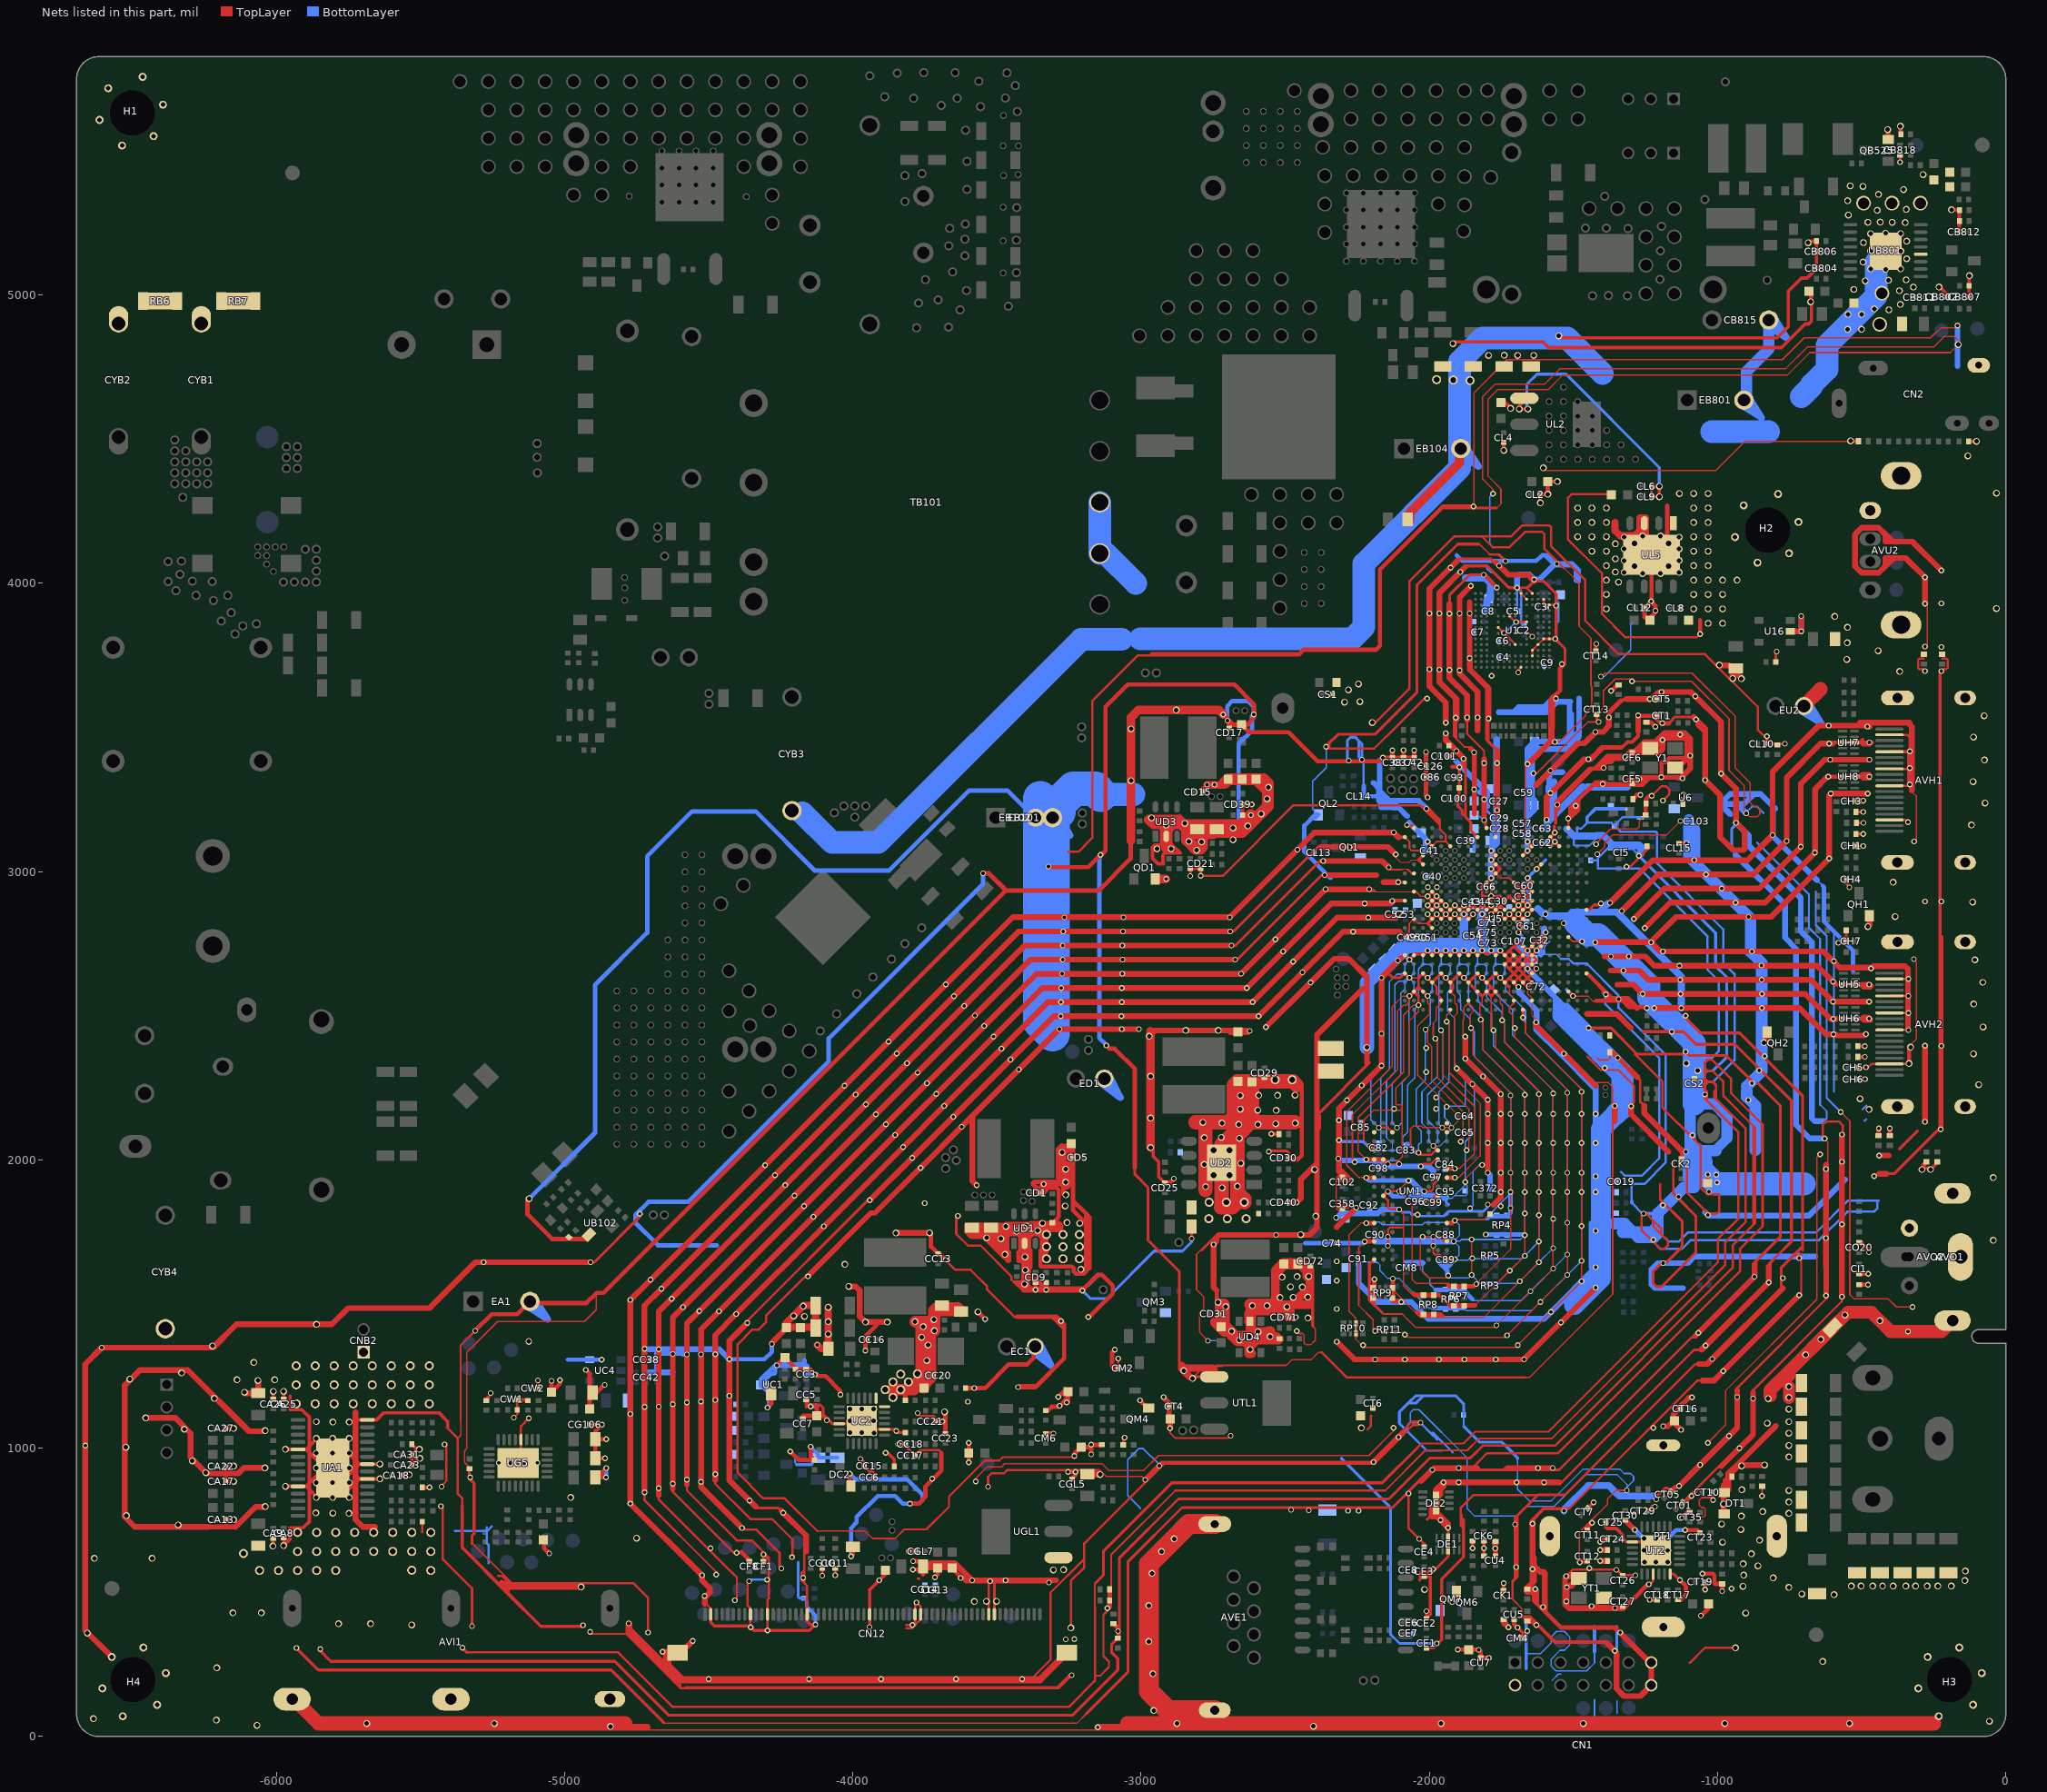
[diagram p0: the nets of this part, all layers, seen from the top]
# Altium PCB MISC84395.PcbDoc (part 16 of 26)
Units mil, origin at the board's own origin, x right, y up, seen from the top; angles counter-clockwise.
Board outline 6692.91 x 5826.77 mil, 2 copper layers (TopLayer, BottomLayer), stack 61.855 mil thick; 951 components, 565 nets, 4374 pads, 1804 vias.
Unrouted connection lines stored in the file: 1.

## Via types
v1: diameter 19.68, hole 11.81, TopLayer to BottomLayer, tented both sides, 1262 vias
v2: diameter 23.62, hole 15.75, TopLayer to BottomLayer, tented both sides, 524 vias
v3: diameter 31.5, hole 19.68, TopLayer to BottomLayer, tented both sides, 11 vias
v4: diameter 24, hole 16, TopLayer to BottomLayer, tented both sides, 6 vias
v5: diameter 19, hole 11.81, TopLayer to BottomLayer, tented both sides, 1 vias

## Nets (pads, with @x,y where several pads share a name; then routed paths per layer and width w, separated by ;. In a path a pad name is that pad's centre, name@x,y a point inside that pad or via, vN(x,y) a via of type N, cw(c..) or ccw(c..) an arc to the next point about the centre after c; other vN are vias at no path point) (continued)
GND: (continued)
  TopLayer w12: v2(-6011.23,661) -6011.23,687.54 CA9.1@-6010.23,688.54 ; CA26.1@-6010.52,1169.98 -6010.52,1196.71 v2(-6010.23,1197) v2@-6009.23,1196 ; v2@-5975.64,663.41 v2(-5974.23,662) ; v2@-5975.23,1196 v2(-5974.23,1197) -5974.17,1196.94 CA25.2@-5974.17,1169.96 ; CA8.1@-5974.23,688.8 v2@-5974.23,662 ; -5952.23,1181.3 -5952.23,1134.04 -5952.19,1134 -5911.57,1134 -5885.23,1107.67 -5885.23,1007.2 ; UA1.24@-5924.23,867.96 -5896.52,867.96 ; UA1.19@-5924.23,995.92 -5896.52,995.92 ; v2@-5858.13,829.58 -5885.23,856.68 ; UA1.EPAD@-5858.13,906.35 -5885.23,879.25 ; UA1.EPAD@-5858.13,957.53 -5885.23,984.63 ; v2@-5858.13,1034.3 -5885.23,1007.2 ; v2(-5804.15,931.94) -5750.17,931.94 -5748.62,930.39 -5737.38,919.15 ; UA1.EPAD@-5750.17,855.17 -5724.67,880.68 -5711.79,893.55 ; UA1.EPAD@-5750.17,906.35 -5737.38,919.15 ; UA1.EPAD@-5750.17,983.12 -5724.67,957.61 -5711.79,944.74 ; -5711.79,1098.28 UA1.14@-5684.07,1098.28 -5651.67,1098.28 -5626.94,1123 -5436.47,1123 -5405.1,1091.63 -5405.1,1074.37 -5406.41,1073.06 ; v2@-5642.04,946.81 v2(-5640.23,945) -5640.5,944.74 UA1.8@-5684.07,944.74 -5711.79,944.74 ; v2@-5640.29,894.06 v2(-5640.23,894) -5640.68,893.55 UA1.6@-5684.07,893.55 -5711.79,893.55 ; CA18.2@-5566.5,906 -5541.23,906 v2(-5539.23,908) -5553.23,908 ; RA21.1@-5529.86,1013.94 -5510.57,994.65 -5513.15,994.65 CA31.2@-5529.86,977.94 CA23.2@-5529.86,941.94 -5511.86,959.94 v2@-5506.56,959.94 ; RA19.1@-5493.86,863.94 -5468.29,863.94 v1(-5468.23,864) ; v1@-5429.23,864 v1(-5426.23,867) ; -5355.07,798.5 -5355.07,655.07 -5195,495 ; -5197.39,537.61 -5196.5,536.72 -5196.5,496.5 -5195,495 ; v1(-4936,386) -4940,382 -5082,382 -5195,495 ; -3941.85,508.15 v1(-3908,542) -3887.19,562.81 CG12.1@-3887.19,577 ; v1(-3886,984) -3883,987 -3882.24,987 -3856.27,961.02 RC26.1@-3856.27,937 ; RM9.2@-3062,1011.73 -3060.5,1013.23 -3060.5,1033.5 v1(-3057.5,1036.5) ; v2(-2967,2043) -2958,2034 -2958,2012.44 -2939,1993.44 -2939,1941.89 CD25.1@-2917,1919.89 ; -2854.76,3123 -2854.76,3140.48 -2866.97,3152.69 -2884.23,3152.69 -2896.44,3140.48 -2896.44,3096.4 -2864.47,3064.43 -2917.66,3064.43 -2924.1,3057.98 -2924.1,3031.15 -2921.62,3028.67 -2921.62,3027 -2941.72,3027 -2960.25,3045.53 -2960.25,3084.07 -2953,3091.32 -2936,3091.32 -2929.56,3097.77 -2929.56,3146.25 -2936,3152.69 -2961.29,3152.69 -2984.16,3175.56 -2984.16,3185 -2977.16,3192 -2868.65,3192 -2866.55,3194.1 -2848,3175.56 pad.VIA5@-2848,3166.69 ; RD16.1@-2829.26,3010.98 CD21.2@-2793.26,3010.97 ; RD27.2@-2647.56,3195.87 CD39.2@-2647.56,3232.87 ; UM1.J2@-2159.73,1875.45 v1(-2143.99,1891.2) ; v1@-2124.91,2899.08 U5.N21@-2084.93,2899.08 ; -2101.84,3119.55 U5.Y21@-2084.93,3119.55 ; -2097.64,2787.76 -2084.93,2775.05 U5.J21@-2084.93,2773.09 ; -2061.17,3158.78 -2060.39,3158 ; C101.2@-1931.91,3399.74 -1924.65,3399.74 v1(-1906.07,3418.31) ; v1(-1921,466) -1906.5,480.5 QM6.E@-1906.5,504 ; -1918.27,3363.45 -1917.48,3363.45 ; v1(-1850,653) R37.1@-1850,678.27 ; DK3.A@-1811,626.73 v1(-1811,653) CK6.1@-1811,678.27 ; CU4.1@-1771,623.73 CU4.1@-1770.01,624.71 ; CL3.2@-1746,4633.81 CL3.2@-1743.32,4633.81 ; CK1.2@-1743,506.74 v1@-1743,530.38 ; v1@-1743,532 v1@-1743,530.38 ; v2@-1742,4461 CL4.2@-1742,4488.26 ; v1(-1741.94,531.44) v1@-1743,530.38 ; CL3.2@-1739.32,4633.81 CL3.2@-1743.32,4633.81 ; v2@-1718.32,4608.81 CL3.2@-1743.32,4633.81 ; v1(-1694.06,378.06) -1677,361 CM4.1@-1677,350 ; CM4.1@-1677,341 CM4.1@-1677,350 ; -1675.5,414.99 -1674.71,414.2 -1670.94,414.2 -1650.8,414.2 v1@-1625.95,389.35 ; UL2.1@-1666.54,4641.55 -1666.54,4637.46 -1688,4616 v2(-1688,4604) v2(-1658,4604) ; v1(-1660,366) -1661,366 CM4.1@-1677,350 ; v1@-1646.5,746.54 -1603.04,790 -1540,790 v1(-1533,783) ; v1@-1634.73,510.73 -1638.17,507.29 -1638.17,496.34 -1638.17,470.88 -1549.69,382.39 -1543.69,376.39 -1535.69,376.39 -1516,376.39 ; v1@-1628.88,392.29 v1@-1625.95,389.35 ; v2(-1615,4279) -1616.26,4280.26 CL2.2@-1616.26,4308 -1590,4308 -1589.19,4308.81 v2(-1589,4309) ; CL1.1@-1589.19,4352 -1556.63,4352 v2(-1555.63,4353) ; -1533.5,547.52 -1533.5,457.65 -1522.35,446.5 -1358.23,446.5 -1334.06,446.5 CT27.1@-1329.29,451.27 -1363,451.27 -1424.96,451.27 -1436.05,451.27 v1(-1437.03,452.26) ; U5.C3@-1518,2584.12 -1517.68,2584.12 v1(-1502.25,2568.68) ; CT7.1@-1450.21,791.79 v1(-1430,812) ; CT14.2@-1422,3764.74 -1422,3789 v1(-1421,3790) ; v1@-1407.46,608.54 v1(-1407,609) ; v1(-1407.29,675) -1398.31,683.98 CT24.2@-1381.81,683.98 ; -1403.38,3431.98 -1402.47,3432.9 -1329.13,3432.9 ; -1399.15,3424.9 -1404.82,3419.23 -1410.48,3419.23 -1416.13,3419.23 -1406.47,3428.9 -1400.81,3428.9 -1333.13,3428.9 -1329.13,3432.9 ; CT25.1@-1388.73,738.27 -1388.73,726.73 -1383.82,721.82 -1351.93,721.82 -1328.48,698.38 -1328.48,687.49 ; -1387.27,327.39 -1563.99,327.39 v1@-1625.95,389.35 ; DU1.A@-1373.79,2372.74 -1364.4,2372.74 -1362.27,2372.74 -1324.43,2334.9 ; -1300.65,3449.75 -1312.28,3449.75 ; -1275.91,3485.74 -1275.91,3470.18 -1296.35,3449.75 -1312.28,3449.75 ; CT29.1@-1241.28,782 CT29.1@-1242.27,783 -1228.27,797 v1(-1217.6,797) ; v1(-1236,474) v1@-1235.54,474.46 ; v1@-1236,474.46 v1@-1235.54,474.46 ; CT1.2@-1210.89,3540 -1210.89,3526.89 -1198,3514 v1@-1193,3514 ; CT18.2@-1210.21,474.46 v1@-1235.54,474.46 ; CL15.1@-1134,3097.73 -1108.58,3097.73 v1(-1108.31,3098) ; CK2.2@-1125,2003.61 -1125,2028.11 -1124.8,2028.31 ; v1(-1124,758) -1124,760.95 -1107.21,777.74 CT35.2@-1097,777.74 ; DA1.A@-1120.27,3235 -1119.24,3236.03 v2(-1119.24,3263.64) v2@-1120,3262.88 ; RS2.2@-1034,1919.22 v1(-1034,1949) ; v1@-1002.41,1922.41 v1(-1002,1922) ; v1@-952.77,513.48 v1(-952.29,513) ; CL10.1@-829.11,3443 CL10.1@-829.11,3445 ; v1@-829.11,3460.27 -829.11,3468.89 v1(-829,3469) ; v2(-539,4494) -537.69,4492.69 DV1.A@-511.61,4492.69 ; DH6.A@-513.89,2357.24 v1(-489.12,2357.24) ; DH5.A@-513.89,2394.24 v1(-489.12,2394.24) ; CH6.1@-513.64,2279.87 v1(-488.37,2279.87) ; v2@-290.91,1966 v2(-291.51,1966.6) -286.11,1972 v2@-256.29,1972 ; v2(-261.69,1966.6) v2@-256.29,1972 ; DV3.A@-238,1993.27 -238,1990.29 v2@-256.29,1972 ; DV2.A@-129.1,4492 v2(-102,4492) ; v2@-5974.23,662 -5952.81,683.42 -5952.81,723.13 -5951.94,724 -5906.7,724 -5885.23,745.47 -5885.23,856.68 ; -5896.52,867.96 -5885.23,856.68 ; -5896.52,867.96 -5885.23,879.25 ; -5896.52,995.92 -5885.23,984.63 ; -5896.52,995.92 -5885.23,1007.2 ; -5885.23,856.68 -5885.23,879.25 ; -5885.23,879.25 -5885.23,984.63 ; -5885.23,984.63 -5885.23,1007.2 ; -5737.38,919.15 -5724.67,906.43 -5711.79,893.55 ; -5737.38,919.15 -5724.67,931.86 -5711.79,944.74 ; -1329.13,3432.9 -1312.28,3449.75 ; v1(-1986.51,2048.68) UM1.D8@-1970.75,2032.93 v1(-1986.51,2048.68)
  TopLayer w13: -6176.94,727.21 -6175.28,728.88 CA13.1@-6175.28,752.06 -6148.29,752.06 v2(-6148.23,752) v2@-6158.23,752 ; CA17.2@-6176,885.16 -6148.39,885.16 v2(-6148.23,885) ; CA27.2@-6175.34,1069 -6148.23,1069 v2@-6150.23,1067 ; CA17.2@-6175.29,885.17 -6175.29,912.21 CA22.1@-6175.29,937.06 -6174.34,938 v2(-6148.23,938) ; v2@-5968.23,998.98 v2(-5968.23,996) -5968.15,995.92 UA1.19@-5924.23,995.92 ; v2@-5966.96,869.27 v2(-5968.23,868) v2(-5968.23,868) UA1.24@-5924.23,867.96 ; v1@-619.19,3328.78 v1(-616.37,3328.78) UH8.GND@-565.81,3328.78 UH8.GND@-524.87,3328.78 -502.81,3328.78 ; v2(-594,3885) v2@-593.1,3884.1 ; CU1.1@-593.1,3806.29 CU1.1@-592.8,3806 ; -592.37,3447.78 UH7.GND@-566.32,3447.78 UH7.GND@-525.37,3447.78 -506.67,3447.78 ; -589.65,2608.02 UH5.GND@-562.81,2608.02 UH5.GND@-521.87,2608.02 -505.71,2608.02 ; -588.65,2489.91 UH6.GND@-562.81,2489.91 UH6.GND@-521.87,2489.91 -502.09,2489.91 ; -497.16,3457.29 -506.67,3447.78 ; -474.37,3339.18 -473.37,3338.18 v1@-473.37,3337.37 ; v1(-474.21,2489.91) -501.84,2489.91 ; v1(-474.21,2608.02) -501.87,2608.02 ; v1(-473.37,3447.78) -502.7,3447.78 ; v1@-471.59,3322.12 -496.16,3322.12 -502.81,3328.78 ; v1@-469.55,3448.75 -464.55,3447.27 -471.59,3440.23 -495.16,3440.23 -502.7,3447.78 ; v1@-468.64,3332.64 v1@-473.37,3337.37 ; -506.67,3447.78 -502.7,3447.78 ; -505.71,2608.02 -501.87,2608.02 ; -505.71,2608.02 -494.57,2596.87 -470.85,2596.87 -464.55,2603.17 -464.55,2603.31 -472.76,2611.52 -498.37,2611.52 -501.87,2608.02 ; -502.81,3328.78 -505.37,3331.34 -505.37,3331.97 -498.16,3339.18 -475.18,3339.18 v1@-473.37,3337.37 ; -502.81,3328.78 v1(-473.37,3328.78) v1@-473.37,3337.37 ; -502.09,2489.91 -501.84,2489.91 ; -502.09,2489.91 -494.16,2481.97 -467.64,2481.97 -467.64,2488.29 -476.23,2496.87 -494.88,2496.87 -501.84,2489.91
  TopLayer w14: RP8.2@-1985.03,1530.97 -1964.14,1530.97 -1926.74,1493.56 RP7.7@-1914.65,1493.56 ; U5.E1@-1455.01,2647.11 -1452.84,2647.11 -1367.58,2561.84 -1310.93,2561.84 -1278.98,2529.9 ; -1421.65,2552.53 -1330.71,2552.53 -1308.07,2529.9 -1283.22,2529.9 -1278.98,2529.9 ; v1(-1245.96,2527.06) -1248.8,2529.9 -1278.98,2529.9
  TopLayer w15: v1(-5310,1407.5) -5253,1464.5 -5164.49,1464.5 -5125.49,1503.5 -4924,1503.5 -4888.5,1539 -4864.64,1539 -3469.64,2934 -3468,2934 -3147.08,2934 -3036.25,3044.84 -3036.25,3104.84 -3034.84,3106.24 ; CC36.2@-5073,682.19 -5070.92,680.11 -5070.92,652.92 v1(-5053,635) ; v1(-5045,1234) CG103.1@-5045,1194.81 -5016,1223.81 v1(-5016,1236) ; v1(-4926,1272) -4913.16,1259.16 CG105.1@-4913.16,1136 ; CG106.1@-4913.27,1082 v1(-4870,1082) -4892.97,1059.03 CG2.2@-4892.97,1031 ; CG104.2@-4902.94,1193 -4888,1193 v1(-4861,1220) ; CG3.2@-4892.97,899 CG3.2@-4887,899 ; v1(-4859,965) CG1.2@-4892.97,965 CG2.2@-4892.97,1031 ; v1(-4856,899) CG3.2@-4887,899 ; v1(-4855,931) CG3.2@-4887,899 ; v1(-4855,1031) CG2.2@-4892.97,1031 ; -4386.26,639.63 -4382,635.37 -4363.95,617.32 CF8.1@-4359,612.37 ; v1(-4296,1141) -4285.06,1151.94 ; CC2.1@-4285.06,1189 -4285.06,1151.94 ; CC2.1@-4282.06,1191 -4282.06,1154.94 -4285.06,1151.94 ; v1@-4260.72,1290.2 -4236.92,1314 -4236.62,1314 CC11.2@-4234.62,1314 -4199.24,1278.62 RC7.2@-4199.24,1273.57 CC3.2@-4162.24,1273.57 ; v1(-4217,989) -4186.46,958.46 RC24.1@-4133,958.46 -4146,971.46 v1(-4146,1005) ; -4173,1112.81 CC4.2@-4125,1112.81 ; CC5.2@-4162,1169.26 -4159.66,1166.92 -4159.66,1153.48 -4155.59,1149.41 ; CC3.2@-4161.92,1273.57 CC3.2@-4162.24,1273.57 ; v1(-4132,1254) v1@-4132,1258.36 ; -4125,1146.91 CC4.2@-4125,1112.81 ; v1(-4090,1097) -4090,1101.25 -4101.56,1112.81 CC4.2@-4125,1112.81 ; v1(-4043,1186) -4043.61,1186 -4043.61,1198.88 -4094.72,1250 -4123.64,1250 v1@-4132,1258.36 ; DC2.3@-4010.5,869 v1(-4010.5,911.5) ; v1(-4006.15,624.47) -4000,630.62 CC1.1@-4000,658.03 ; v1(-3956,1339) -3956,1362 ; CC16.1@-3956,1386 CC16.1@-3956,1377 ; -3951.25,1366.75 -3956,1362 ; -3918,1437.72 -3918,1427 -3956,1389 CC16.1@-3956,1377 ; RC17.1@-3817.73,1166 -3817.73,1202.66 ; v1(-3807,642) CGL7.2@-3781.57,642 ; v1(-3802,807.66) -3771.75,807.66 -3748.5,830.9 -3748.5,866.39 v1@-3725,889.89 ; v1(-3792,579) -3766.97,579 CC19.2@-3755.97,590 ; v1(-3791,608) -3773.97,608 CC19.2@-3755.97,590 ; -3782.39,1209 CC22.2@-3753.62,1209 CC22.2@-3742.62,1209 ; pad.VIA5@-3772,1252 -3763.14,1252 -3730.86,1252 CC20.1@-3720.73,1252 ; -3755.97,561.73 CC19.2@-3755.97,590 ; CC19.2@-3750.16,584.19 CGL6.2@-3705,584.19 ; v2@-3732.83,1747.1 -3732.73,1747 -3729.23,1743.5 -3729.23,1698.96 CC13.1@-3704,1673.73 -3699.05,1673.73 v1(-3678.31,1652.99) ; v1(-3725,894) v1@-3725,889.89 ; v1(-3715,552) -3715,554 -3705,564 CGL6.2@-3705,584.19 ; -3692.9,983 -3692.9,921.98 -3700.23,914.66 v1@-3725,889.89 ; v2(-3682,1126) -3679,1123 -3679,1083 CC23.1@-3679,1050.46 ; RC18.1@-3608.54,1208.27 v1(-3579.27,1208.27) -3541.81,1208.27 -3459.42,1290.66 -3395,1290.66 -3372.79,1312.87 EC1.2@-3372.79,1353 ; v1(-3597.81,951.19) CM9.1@-3597.81,984 v1(-3597.81,1018.81) ; v2(-3566,1473) v1(-3541,1448) ; -3430,1456 -3307,1456 ; -3404.41,1743 -3402.4,1743 -3388.94,1743 ; v2@-3401.15,1571.85 -3383.48,1554.17 ; -3379.4,1766 -3376.91,1768.5 -3364.41,1781 -3306.36,1781 -3285.66,1801.7 -3285.66,1895.77 -3292.98,1903.09 -3323.02,1903.09 -3330.34,1895.77 -3330.34,1892.99 -3340.67,1882.66 -3358.53,1882.66 -3358.53,1900.02 -3365.85,1907.34 -3367.42,1907.34 -3375.04,1914.96 -3375.04,1920.1 -3371,1924.14 -3301.14,1924.14 -3300,1923 ; v1@-3366,1549 v1(-3366,1550) v1@-3366,1554.17 ; CD9.2@-3366,1575.54 v1@-3366,1554.17 ; CD1.1@-3349.43,1884 CD1.1@-3349.43,1889.35 ; -3335.49,1904.59 -3337.88,1904.59 v1@-3343.64,1910.36 ; v1@-3331.18,1917.18 v1@-3330,1916 ; CM6.1@-3331,1050.73 v1(-3304.27,1050.73) ; RM3.2@-3331,1130.73 -3322.91,1130.73 -3309.92,1143.72 -3286.28,1143.72 v1(-3283,1147) -3253.81,1176.19 ; -3330,539 v1(-3524,539) -3607.95,539 -3618.95,550 v1(-3626,550) -3626,554.19 CGL49.2@-3656,584.19 CGL6.2@-3705,584.19 ; v1@-3329,1549 v1(-3329,1550) ; RD4.1@-3329,1575.54 v1@-3329,1554.17 ; v1(-3321,3018) v1@-3318,3015 ; v1@-3318.78,3015 v1@-3318,3015 ; v1(-3287,1178) -3269,1196 CM3.1@-3253.81,1196 -3253.81,1176.19 ; -3275,2051 -3288.64,2037.36 -3288.64,1937 -3274.64,1923 ; v2@-3270,1881 v2@-3270,1916 ; -3267,1344 -3267,1416 ; v2@-3262,1916 v2@-3270,1916 ; v2(-3262,1923) -3274.64,1923 ; -3262,2037.19 CD8.1@-3242,2057.19 ; v1(-3258,1159) -3254.21,1159 -3253.81,1159.4 -3253.81,1176.19 ; v1(-3253.5,917.5) v1(-3227.5,917.5) -3227.5,907 -3239,895.5 CGL5.2@-3239,892.74 ; CD8.1@-3236.5,2051.69 -3236.5,1859.17 ; -3232.66,1620.44 -3232.66,1611 ; v1(-3231.43,973.34) -3231.43,980.76 CM7.1@-3208.19,1004 v1@-3173,1004 ; -3229,1547 v1(-3204,1547) ; v2(-3209,1620) -3195.5,1620 -3191.5,1624 ; v1(-3183,1455) -3179.33,1455 -3157.67,1476.67 ; -3173.33,1461 -3157.67,1476.67 ; v1(-3173,978.5) v1(-3173,1012.5) ; v1@-3165,1012 R28.1@-3136,1012 ; v1(-3141,3058) -3184,3015 v1@-3318,3015 ; v1@-3140.64,3055 -3123.34,3072.3 -3123.34,3571.64 -3046.49,3648.5 -2676.5,3648.5 -2609,3581 v1(-2609,3545) -2609,3532 -2632,3509 CD20.2@-2651,3509 ; v1(-3120,2397) -3108.66,2385.66 -3091.44,2385.66 -3021.5,2315.71 -3021.5,1972 ; v1(-3117.49,445.33) -3109.27,453.55 DI4.A@-3109.27,510 ; DI2.A@-3096,391.27 -3080,375.27 v1(-3080,365.5) ; v1(-3091,1342) -3101,1332 -3101,1286 -3092,1277 CM2.2@-3079.74,1277 ; v1(-3003.5,1166) -2976,1138.5 QM4.E@-2973,1138.5 ; -2963,3753.5 -2520,3753.5 ; v1(-2936.63,938.81) -2936.63,942.35 -2929.48,949.5 -2196.02,949.5 v1(-2193.52,952) ; CD25.1@-2917,1919.89 -2901.11,1919.89 v1(-2886,1935) ; CD15.2@-2786.27,3276 -2786.27,3285.73 v1(-2771,3301) ; -2738.65,1547.77 -2737.66,1546.78 -2737.66,1494.66 ; v1(-2715,3545) -2700,3530 v1(-2700,3523.19) ; CD17.2@-2694,3497.76 -2694,3523.19 -2679.81,3509 CD20.2@-2651,3509 ; RD27.2@-2647.56,3195.87 v1(-2619.13,3195.87) ; CD39.2@-2647.56,3232.87 v1(-2616.13,3232.87) ; v1(-2548,2090) D12.A@-2521.73,2090 ; -2511.5,3753.5 -2520,3753.5 ; CD40.2@-2488.27,1852 v1(-2461,1852) ; CD30.2@-2488.26,2006 -2483.92,2001.66 -2456.75,2001.66 -2443.07,2015.33 -2443.07,2248.07 -2463,2268 ; v1(-2234,3388) v1@-2239.5,3382.5 ; v1(-2218.79,1938.44) UM1.G1@-2191.23,1938.45 ; v1(-2218.79,2001.43) UM1.E2@-2159.73,2001.44 v1(-2143.99,1985.69) ; v1(-2206.98,2048.68) UM1.D1@-2191.23,2032.93 ; v1(-2128,3420) v1(-2128,3420) C38.1@-2128.06,3394.79 ; RP9.1@-2126.76,1549.17 v1(-2126.76,1588.54) ; v1(-2090.06,3421.06) C37.1@-2090.06,3394.79 ; v1(-2053.06,3420.06) C42.1@-2053.06,3394.79 C37.1@-2090.06,3394.79 ; v1@-2011.38,3415 C126.2@-2011.38,3365.74 C86.2@-2011.38,3327.74 -2011.38,3262.67 v1(-2006.19,3257.47) ; -1920.4,3363.45 -1918.27,3363.45 ; -1917.48,3363.45 -1881.48,3363.45 v1(-1881.48,3390.91) ; v1@-1904.38,301.62 v1(-1901.38,301.62) CU6.2@-1864,301.62 -1828.62,301.62 -1822,295 CU7.2@-1822,272.57 v1(-1793.57,272.57) ; v1(-1847.11,4266.84) -1952.44,4266.84 -2171.38,4047.91 -2171.38,3782.08 -2183.96,3769.5 -2435.69,3769.5 -2451.69,3753.5 -2520,3753.5 ; v1(-1811.34,4029.43) -1809.08,4029.43 -1766,3986.35 v1(-1766,3984.27) ; v1(-1771.67,652) -1771,651.33 CU4.1@-1771,626.73 ; -1735.9,928.5 -1730.9,933.5 -1574.5,933.5 v1(-1572,931) ; CU5.1@-1706.35,406.16 -1706.35,390.35 v1(-1694.06,378.06) ; -1645.52,403.27 -1641.98,403.27 ; v2@-1589.19,4308.81 CL1.1@-1589.19,4352 ; -1568.07,3607.16 -1546.49,3628.74 -1546.49,3704.9 v1@-1531.71,3719.68 ; v1(-1556.65,3231.74) -1556.65,3233.01 -1556.65,3243.61 -1443.02,3357.24 -1435.95,3357.24 ; -1553.15,3219.17 -1553.15,3236.55 -1553.15,3240.04 -1549.29,3243.9 -1435.95,3357.24 ; -1527.5,543.75 -1527.5,471.22 v1(-1524.71,468.43) ; v1(-1518.65,3183.74) -1518,3183.09 -1517.65,3182.74 -1514.98,3182.74 -1514.98,3193.65 -1511.15,3197.49 ; v1(-1478,604) -1473.46,608.54 CT12.1@-1452,608.54 ; CT11.1@-1452,716.26 -1452,725 v1@-1437,740 ; -1431,3301.09 -1431.78,3301.09 ; v1(-1398.65,3303.74) -1398.65,3301.58 v1@-1398.15,3301.08 ; v1(-1395.33,3359.58) v1@-1393.49,3359.58 ; -1385.77,325.89 -1383.27,323.39 ; -1377.21,3545.75 -1377.21,3552.44 -1336.74,3592.91 -1332.84,3592.91 ; v1@-1367.8,3626.83 -1346.9,3647.73 D13.A@-1343,3647.73 ; -1364.4,2372.74 -1304.9,2313.24 ; v1@-1363,451.27 -1358.23,446.5 -1354.73,443 -1326.88,443 -1318.61,451.27 -1311,458.88 -1284.88,485 ; -1302.83,2174.5 v1@-1300.33,2177 ; CF5.2@-1296.64,3305 CF5.2@-1291,3305 ; L3.2@-1294.31,3250.74 -1278.31,3266.74 -1268.77,3266.74 v1(-1267.77,3265.74) ; CF6.2@-1291.57,3418.41 -1303.31,3418.41 v1@-1321.32,3400.4 ; v1@-1274.17,3540 CT1.2@-1210.89,3540 ; R3.1@-1249.77,3196.47 D4.A@-1249.77,3234.47 ; D4.A@-1248.5,3235.74 -1248.5,3251.64 -1237.4,3262.74 v1(-1228.77,3262.74) ; D14.A@-1248,3517.46 -1231.46,3517.46 v1(-1216,3502) ; UL5.EPAD@-1244.2,4155 UL5.EPAD@-1229.2,4140 ; v1@-1236,3598 -1230,3598 CT5.1@-1210.73,3598 -1210.73,3617.27 -1205.16,3622.84 v1(-1195,3622.84) ; Y1.4@-1234.65,3428.97 Y1.4@-1234.65,3428.74 ; v1@-1229.2,3939.26 UL5.EPAD@-1229.2,4098.55 -1229.2,4115.17 -1174.7,4169.67 -1174.7,4269.18 ; v1(-1195.09,3327.09) v1@-1195.59,3326.59 ; v1@-1193,3514 v1@-1191,3514 ; v1(-1192,3515) v1@-1191,3514 ; v1(-1191.15,3456.24) -1191.15,3454.98 -1195.52,3450.61 -1196.78,3450.61 -1211.71,3450.61 Y1.4@-1234.65,3427.67 ; -1168.83,3514 v1@-1191,3514 ; CT05.1@-1162.17,850.83 -1147.31,865.68 v1@-1142.34,865.68 ; CT17.1@-1138.21,474.47 -1127.53,474.47 -1110,492 -1110,522 v1(-1131,543) ; v1@-1127.5,3325.02 -1129.06,3326.59 v1@-1195.59,3326.59 ; CT01.1@-1121.17,812.83 -1115.5,812.83 -1075.25,853.08 ; -1116.25,3466.08 -1125.91,3475.74 v1(-1130.15,3475.74) -1187.65,3475.74 Y1.4@-1234.65,3428.74 ; v1(-1113,716) -1070.05,716 CT23.2@-1061.25,707.2 ; -1107.97,3404.5 -1107.97,3400.84 -1115.3,3393.52 -1168.45,3393.52 -1182.26,3379.7 -1194.15,3379.7 -1194.59,3379.26 -1194.59,3333.91 v1@-1201.91,3326.59 ; v1(-1060.84,3824) -1060.84,3871.83 ; v1(-1058,419) -1031.19,445.81 CT8.2@-1031.19,460 ; v1(-1053,565) -1017,565 -1012,560 -1012,533 -1008.27,529.27 LT5.1@-984,529.27 ; CT19.2@-1043.26,536 -1043.26,510.26 v1(-1043,510) ; LT5.1@-992.27,529.27 LT5.1@-984,529.27 ; v1(-984,504) LT5.1@-984,529.27 ; DO7.A@-509,1567.46 v1(-478.46,1567.46) ; CI1.1@-509.01,1604.97 v1(-477.44,1604.97) ; CO20.1@-508.99,1713 -502.79,1712.99 -475,1685.2 v1(-475,1679.53) ; DU9.A@-442,2083.73 -442,2108 v1(-441,2109) ; v2(-410,5573) -409,5572 QB525.E@-409,5538.5 ; DU8.A@-403,2083.73 v1(-403,2109) ; v2(-366,5585) -366,5558.27 RB834.1@-364.73,5557 ; v2(-336,2334) -336,2386 v2(-331,2391) ; v2@-286.11,1972 -286.11,1983.16 DV4.A@-276,1993.27 ; CC3.2@-4162.24,1273.57 -4147.21,1273.57 v1@-4132,1258.36 ; -3956,1362 CC16.1@-3956,1377 ; -3413.79,1554.17 -3406.62,1547 -3376.31,1547 ; -3413.79,1554.17 -3433.52,1573.9 -3415.98,1573.9 -3412.48,1577.4 -3408.65,1581.23 -3408.65,1642.76 -3415.98,1650.09 -3424.9,1650.09 -3424.9,1680.11 -3419.06,1685.96 -3419.06,1735.68 -3428.88,1745.5 -3429.5,1746.12 -3429.5,1755.5 -3421.2,1755.5 -3418.64,1752.94 -3392.46,1752.94 -3388.94,1752.94 -3388.94,1743 ; -3413.79,1554.17 -3383.48,1554.17 ; -3388.94,1743 -3386.46,1743 -3355.02,1743 -3344.26,1732.24 -3344.26,1691.72 -3349.1,1686.88 -3349.1,1632 -3347.46,1630.36 -3242.58,1630.36 -3239.98,1630.35 -3232.66,1623.03 -3232.66,1611 ; -3388.94,1743 -3388.94,1740.52 -3388.94,1691.72 -3384.1,1686.88 -3384.1,1627.28 -3388.34,1623.04 -3388.34,1594.96 -3381.02,1587.64 -3366.64,1587.64 v1@-3333.17,1554.17 ; -3383.48,1554.17 -3376.31,1547 ; -3383.48,1554.17 v1@-3366,1554.17 ; -3376.31,1547 v1(-3204,1547) ; v1@-3366,1554.17 v1@-3333.17,1554.17 ; CD1.1@-3349.43,1889.35 -3349.43,1904.57 v1@-3343.64,1910.36 ; CD1.1@-3349.43,1889.35 -3348.43,1888.35 -3348.43,1885 CD1.1@-3346.43,1885 -3345.11,1885 -3314.11,1916 ; v1@-3343.64,1910.36 v1(-3338,1916) v1@-3330,1916 ; v1@-3343.64,1910.36 -3335.64,1910.36 v1@-3330,1916 ; v1@-3333.17,1554.17 v1(-3329,1550) ; v1@-3333.17,1554.17 v1@-3329,1554.17 ; v1@-3330,1916 -3314.11,1916 ; v1(-3329,1550) v1@-3329,1554.17 ; v1@-3329,1554.17 -3196.83,1554.17 ; -3314.11,1916 -3307.11,1923 -3300,1923 ; -3314.11,1916 -3293,1916 ; -3307,1456 -3267,1416 ; -3307,1456 -3293,1456 v1(-3278.23,1441.23) -3267,1430 -3267,1416 ; -3300,1923 -3293,1916 ; -3300,1923 -3274.64,1923 ; -3293,1916 v2@-3270,1916 ; -3274.64,1923 -3270,1918.36 v2@-3270,1916 ; -3267,1311.18 -3366.18,1212 v1(-3427,1212) -3424.34,1214.66 -3363.52,1214.66 -3267,1311.18 ; -3267,1311.18 -3267,1416 ; -3236.5,1859.17 -3191.5,1814.17 ; -3236.5,1859.17 -3236.5,1825.17 -3192.17,1780.83 -3192.17,1770.67 -3191.5,1770 ; -3232.66,1611 -3226.66,1605 -3199.33,1605 -3179.5,1624.83 -3179.5,1636 ; v1(-3204,1547) -3196.83,1554.17 ; -3196.83,1554.17 -3150,1601 -3135.17,1601 -3135.17,1600 -3098.42,1563.25 -3098.42,1535.91 -3157.67,1476.67 ; -3191.5,1624 -3179.5,1636 ; -3191.5,1624 -3191.5,1770 ; -3191.5,1770 -3191.5,1814.17 ; -3191.5,1814.17 -3179.5,1802.17 -3179.5,1636 ; CD20.2@-2651,3509 -2625.69,3483.69 -2489.16,3483.69 -2387.97,3382.5 v1@-2239.5,3382.5 ; v1@-2239.5,3382.5 -2173.5,3382.5 v1(-2161.21,3394.79) C38.1@-2128.06,3394.79 ; C38.1@-2128.06,3394.79 C37.1@-2090.06,3394.79 ; -1511.15,3197.49 -1511.15,3186.57 -1483.15,3214.57 -1483.15,3231.74 ; -1511.15,3197.49 -1511.15,3203.74 ; -1511.15,3203.74 -1511.15,3221.73 -1483.15,3249.73 ; -1511.15,3203.74 -1483.15,3231.74 ; -1483.15,3231.74 -1483.15,3249.73 ; -1483.15,3249.73 -1455.51,3277.36 ; -1455.51,3277.36 -1431.78,3301.09 ; -1455.51,3277.36 -1454.74,3277.36 -1431.01,3301.08 v1@-1398.15,3301.08 ; -1435.95,3357.24 -1426.5,3357.24 ; -1431.78,3301.09 -1422.63,3310.24 -1391.26,3310.24 -1384.67,3303.65 -1318.63,3303.65 -1311.3,3310.97 -1311.3,3317.11 -1281.62,3317.11 -1272.15,3326.59 v1@-1269.41,3326.59 ; -1426.5,3357.24 -1383.35,3400.4 -1366.99,3400.4 ; -1426.5,3357.24 -1410.15,3357.24 ; -1410.15,3357.24 v1@-1393.49,3357.24 ; -1410.15,3357.24 -1366.99,3400.4 ; v1@-1398.15,3301.08 CF5.2@-1294.92,3301.08 ; v1@-1393.49,3357.24 -1391.99,3358.74 -1392.83,3359.58 v1@-1393.49,3359.58 ; v1@-1393.49,3357.24 v1@-1393.49,3359.58 ; v1@-1393.49,3359.58 -1393.49,3371.01 -1384.67,3379.83 -1370.21,3379.83 -1358.8,3391.24 -1329.15,3391.24 v1(-1322.33,3398.06) -1322.33,3399.39 v1@-1321.32,3400.4 ; -1366.99,3400.4 v1@-1321.32,3400.4 ; v1@-1321.32,3400.4 -1300.6,3400.4 -1287.8,3413.2 -1273.33,3427.67 Y1.4@-1234.65,3427.67 ; CF5.2@-1294.92,3301.08 -1272,3301.08 ; CF5.2@-1294.92,3301.08 CF5.2@-1291,3305 ; CF5.2@-1291,3305 -1281,3305 -1274,3312 ; -1274,3312 -1274,3322 v1@-1269.41,3326.59 ; -1274,3312 -1259.41,3326.59 ; -1272,3301.08 -1261.25,3301.08 -1237.59,3324.74 -1197.43,3324.74 v1@-1195.59,3326.59 ; -1272,3301.08 -1272,3303 -1248.41,3326.59 ; v1@-1269.41,3326.59 -1259.41,3326.59 ; -1259.41,3326.59 -1248.41,3326.59 ; -1248.41,3326.59 v1@-1201.91,3326.59 ; Y1.4@-1234.65,3427.67 Y1.4@-1234.65,3428.74 ; v1@-1201.91,3326.59 v1@-1195.59,3326.59 ; -1253.47,3883.07 -1242.39,3872 -1216.2,3898.19 v1(-1216.2,3905) -1216.2,3922 v1(-1231.2,3937) -1231.47,3937 CL12.2@-1253.47,3915 -1253.47,3883.07